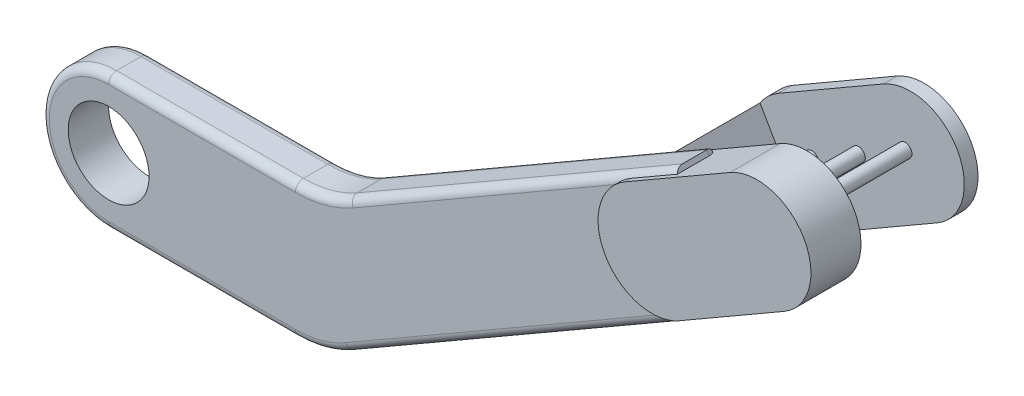
SolidWorks part; units mm, degrees
ref_plane "Front Plane" through (0, 0, 0) normal (0, 0, 1) x (1, 0, 0)
ref_plane "Top Plane" through (0, 0, 0) normal (0, 1, 0) x (1, 0, 0)
ref_plane "Right Plane" through (0, 0, 0) normal (1, 0, 0) x (0, 0, -1)
other "Configuration Table"
sketch "Sketch1" plane through (0, 0, 0) normal (0, 0, 1) x (1, 0, 0)
  line L0 (0, 0) -> (80, 0) construction
  line L1 (0, 25) -> (69.282, 25)
  line L2 (0, -25) -> (69.282, -25)
  line L3 (89.282, 30.359) -> (209.9038, 100)
  line L4 (89.282, -19.641) -> (231.5544, 62.5)
  line L5 (209.9038, 100) -> (231.5544, 62.5) construction
  line L6 (209.9038, 100) -> (231.5544, 62.5)
  arc A0 (0, 25) -> (0, -25) centre (0, 0) ccw
  arc A1 (69.282, 25) -> (89.282, 30.359) centre (69.282, 65) ccw
  arc A2 (69.282, -25) -> (89.282, -19.641) centre (69.282, 15) ccw
  point P3 (40, 0)
  point P11 (80, 25)
  point P15 (80, -25)
  dimension "D1" = 25
  dimension "D3" = 150
  dimension "D6" = 40
  dimension "D2" = 80
  dimension "D4" = 150
  dimension "D5" = 43.3013
extrude "Boss-Extrude1" add sketch "Sketch1" along normal blind 15
fillet "Fillet1" radius 3 15 edges at (149.5929, 65.1795, 15) (79.6348, 26.363, 15) (160.4182, 21.4295, 15) (79.6348, -23.637, 15) (34.641, -25, 15) (-25, 0, 15) (34.641, -25, 0) (79.6348, -23.637, 0) (160.4182, 21.4295, 0) (220.7291, 81.25, 0) (149.5929, 65.1795, 0) (79.6348, 26.363, 0) (34.641, 25, 0) (-25, 0, 0) (34.641, 25, 15)
sketch "Sketch2" plane through (0, 0, 15) normal (0, 0, 1) x (1, 0, 0)
  circle A0 centre (0, 0) radius 15
  dimension "D1" = 30
extrude "Cut-Extrude1" cut sketch "Sketch2" against normal through all
sketch "Sketch3" plane through (0, 0, 0) normal (0, 0, -1) x (-1, 0, 0)
  line L0 (-242.5532, 93.7221) -> (-203.582, 71.2221) construction
  line L1 (-232.5532, 111.0427) -> (-193.582, 88.5427)
  line L2 (-252.5532, 76.4016) -> (-213.582, 53.9016)
  line L3 (-227.4564, 63.5981) -> (-87.782, -17.0429) construction
  arc A0 (-232.5532, 111.0427) -> (-252.5532, 76.4016) centre (-242.5532, 93.7221) ccw
  arc A1 (-213.582, 53.9016) -> (-193.582, 88.5427) centre (-203.582, 71.2221) ccw
  point P2 (-223.0676, 82.4721)
  dimension "D1" = 20
  dimension "D2" = 45
extrude "Boss-Extrude2" add sketch "Sketch3" along normal blind 45 and the other way blind 17 contours L2 A1 L1 A0
sketch "Sketch4" plane through (10.0554, -17.4165, 0) normal (-0.5, 0.866, 0) x (0.866, 0.5, 0)
  line L1 (239.4586, 15.1298) -> (313.4633, 15.1298)
  line L2 (239.4586, 15.1298) -> (239.4586, -15.8584)
  line L3 (239.4586, -15.8584) -> (313.4633, -15.8584)
  line L4 (313.4633, 15.1298) -> (313.4633, -15.8584)
  line L5 (276.461, -15.8584) -> (276.461, 15.1298) construction
  line L6 (239.4586, -0.3643) -> (313.4633, -0.3643) construction
  point P96 (276.461, -0.3643)
sketch "Sketch6" plane through (10.0554, -17.4165, 0) normal (-0.5, 0.866, 0) x (0.866, 0.5, 0)
  line L1 (202.7611, 39.8997) -> (286.3778, 39.8997)
  line L2 (202.7611, 39.8997) -> (202.7611, 1.5661)
  line L3 (202.7611, 1.5661) -> (286.3778, 1.5661)
  line L4 (286.3778, 39.8997) -> (286.3778, 1.5661)
  line L5 (244.5694, 1.5661) -> (244.5694, 39.8997) construction
  line L6 (202.7611, 20.7329) -> (286.3778, 20.7329) construction
  point P292 (244.5694, 20.7329)
extrude "Cut-Extrude3" cut sketch "Sketch6" against normal through all
sketch "Sketch8" plane through (0, 0, -39.8997) normal (0, 0, 1) x (1, 0, 0)
  circle A0 centre (240.6389, 93.8261) radius 2.5
  dimension "D1" = 5
extrude "Boss-Extrude3" add sketch "Sketch8" along normal blind 38
pattern_linear "LPattern1" count 3 spacing 20 along (-0.866, -0.5, 0) of "Boss-Extrude3"
